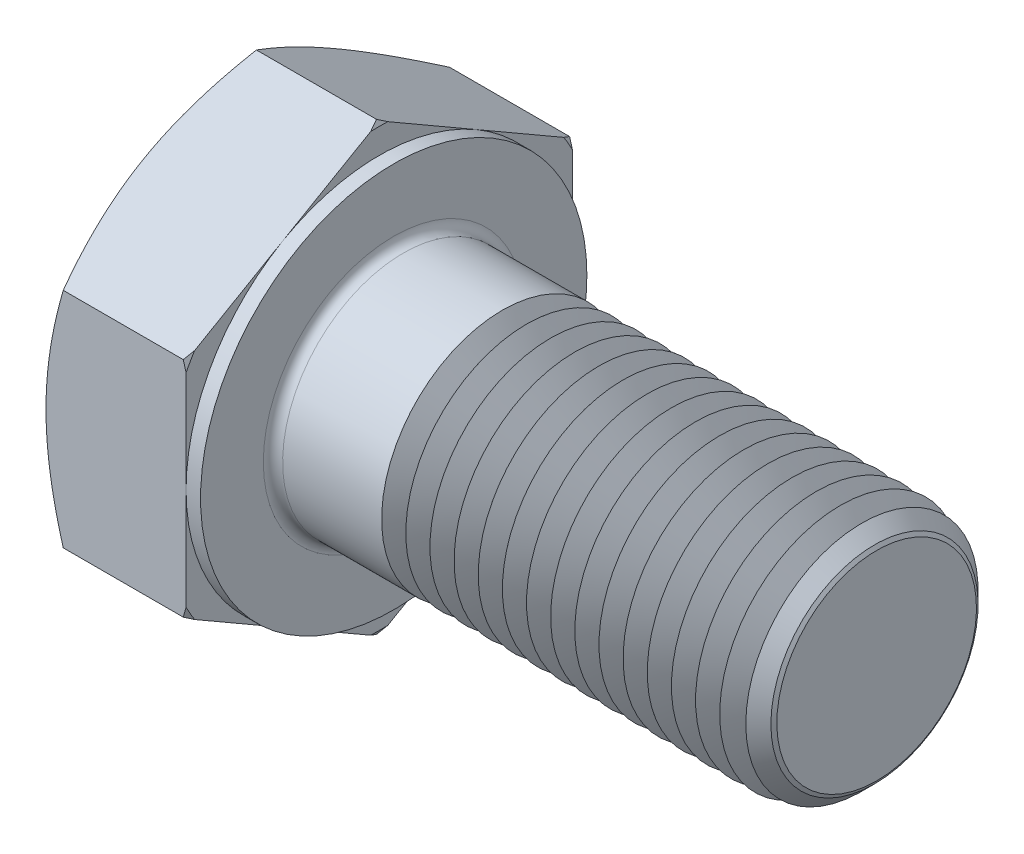
from build123d import *

# Parameters (mm, degrees)
EXTRUDE_393_DEPTH      = 6.4
SKETCH_4_W             = 0.6
SKETCH_4_H             = 11.237604307
CHAMFER_2074_SIZE      = 0.8
FILLET_2119_R          = 0.4
PATTERN_LINEAR_1_COUNT = 16
PATTERN_LINEAR_1_PITCH = 1


with BuildPart() as part:
    # 草图1 → Extrude 393 (new body)
    with BuildSketch(Plane(origin=(0, 0, 0), x_dir=(0, 0, -1), z_dir=(1, 0, 0))):
        Polygon((8, 4.618802154), (8, -4.618802154), (0, -9.237604307), (-8, -4.618802154), (-8, 4.618802154), (0, 9.237604307), align=None)
    extrude(amount=EXTRUDE_393_DEPTH)

    # 草图2 → 凸台-旋转1 (revolve)
    with BuildSketch(Plane.XY, mode=Mode.PRIVATE) as revolve_1_sk:
        Polygon((0, 0), (26.4, 0), (26.4, 4.134), (26.4, 5), (0, 5), align=None)
    revolve(revolve_1_sk.sketch.rotate(Axis((0, 0, 0), (1, 0, 0)), 90), axis=Axis((0, 0, 0), (1, 0, 0)))

    # 草图3 → 切除-旋转1 (revolve, cut)
    with BuildSketch(Plane.XY):
        Polygon((0, 8), (3.601282526, 14.237604307), (3.601282526, 19.237604307), (-10, 19.237604307), (-10, 8), align=None)
    revolve(axis=Axis((0, 0, 0), (1, 0, 0)), mode=Mode.SUBTRACT)

    # 草图5 → 切除-旋转2 (revolve, cut)
    with BuildSketch(Plane.XY):
        Polygon((6.4, 8), (2.798717474, 14.237604307), (2.798717474, 19.237604307), (12.798717474, 19.237604307), (12.798717474, 8), align=None)
    revolve(axis=Axis((0, 0, 0), (1, 0, 0)), mode=Mode.SUBTRACT)

    # 草图4 → 切除-旋转3 (revolve, cut)
    with BuildSketch(Plane.XY, mode=Mode.PRIVATE) as cut_revolve_3_sk:
        with Locations((6.1, 13.618802154)):
            Rectangle(SKETCH_4_W, SKETCH_4_H)
    revolve(cut_revolve_3_sk.sketch.rotate(Axis((0, 0, 0), (1, 0, 0)), 270), axis=Axis((0, 0, 0), (1, 0, 0)), mode=Mode.SUBTRACT)

    # Chamfer 2074
    chamfer_2074_edges = [part.edges().sort_by_distance(p)[0] for p in [
        (26.4, 0, -5),
    ]]
    chamfer(chamfer_2074_edges, length=CHAMFER_2074_SIZE)

    # Fillet 2119
    fillet_2119_edges = [part.edges().sort_by_distance(p)[0] for p in [
        (6.4, 0, -5),
    ]]
    fillet(fillet_2119_edges, radius=FILLET_2119_R)

    # 草图6 → 切除-旋转4 (revolve, cut)
    with BuildSketch(Plane.XY):
        Polygon((11.4, -4.134), (10.900014667, -5), (10.900014667, -6.25), (11.899985333, -6.25), (11.899985333, -5), align=None)
    cut_revolve_4 = revolve(axis=Axis((-3.175, 0, 0), (1, 0, 0)), mode=Mode.SUBTRACT)

    # 阵列(线性)1: 切除-旋转4 ×16
    with Locations(*[(i * PATTERN_LINEAR_1_PITCH, 0, 0) for i in range(1, PATTERN_LINEAR_1_COUNT)]):
        add(cut_revolve_4, mode=Mode.SUBTRACT)


solid = part.part
